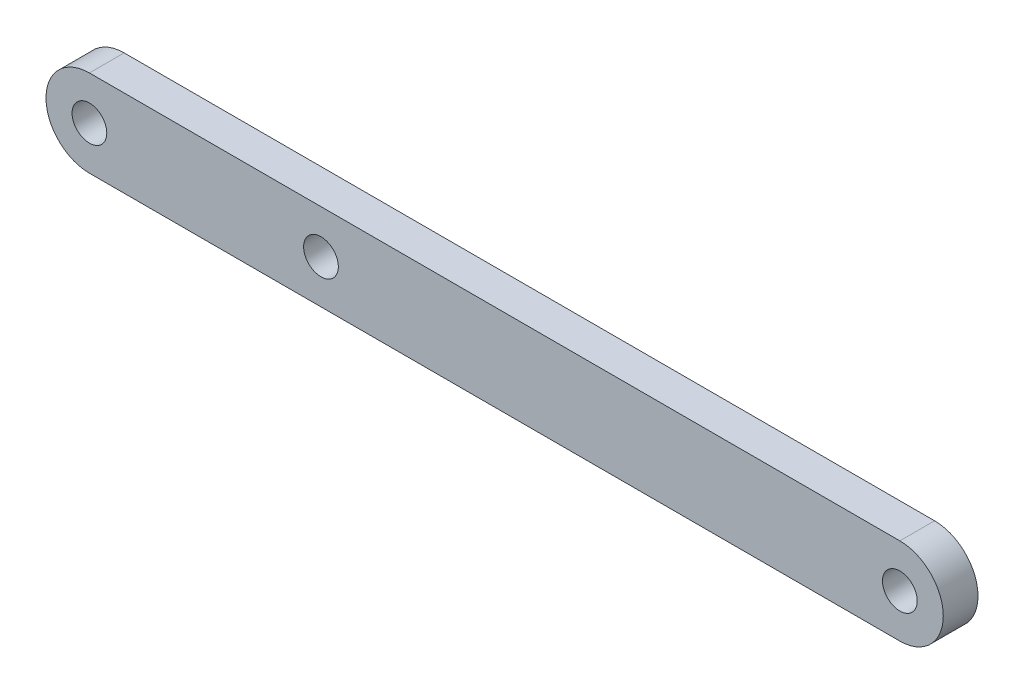
SolidWorks part; units mm, degrees
ref_plane "Front Plane" through (0, 0, 0) normal (0, 0, 1) x (1, 0, 0)
ref_plane "Top Plane" through (0, 0, 0) normal (0, 1, 0) x (1, 0, 0)
ref_plane "Right Plane" through (0, 0, 0) normal (1, 0, 0) x (0, 0, -1)
other "Configuration Table"
sketch "Sketch1" plane through (0, 0, 0) normal (0, 0, 1) x (1, 0, 0)
  line L0 (0, 0) -> (140, 0) construction
  line L1 (0, 7.5) -> (140, 7.5)
  line L2 (0, -7.5) -> (140, -7.5)
  circle A0 centre (0, 0) radius 3
  circle A1 centre (40, 0) radius 3
  circle A2 centre (140, 0) radius 3
  arc A3 (0, 7.5) -> (0, -7.5) centre (0, 0) ccw
  arc A4 (140, -7.5) -> (140, 7.5) centre (140, 0) ccw
  dimension "D1" = 6
  dimension "D2" = 140
  dimension "D3" = 40
  dimension "D4" = 15
  dimension "D5" = 15
extrude "Boss-Extrude1" add sketch "Sketch1" along normal blind 6
